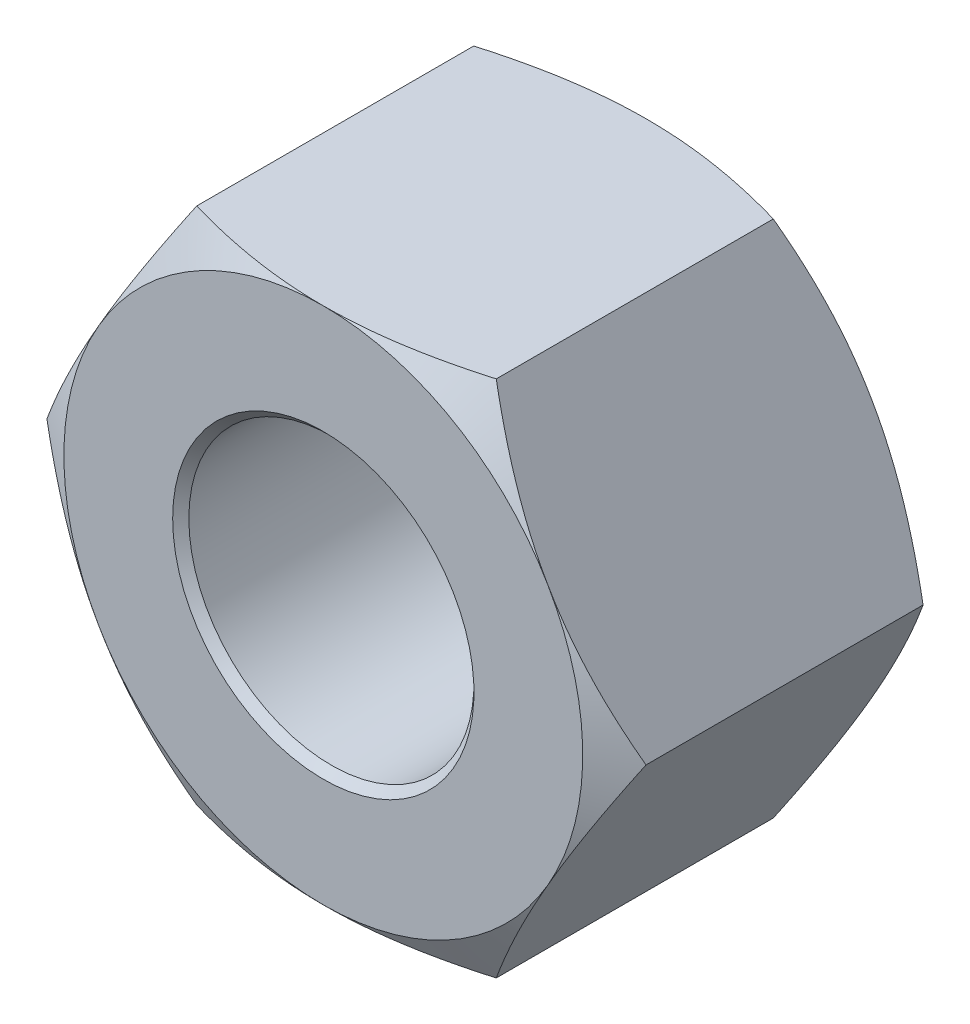
from build123d import *

# Parameters (mm, degrees)
SKETCH1_R          = 4.188125
BOSS_EXTRUDE_DEPTH = 9.5
SKETCH2_OUTSIDE_W  = 80.144
SKETCH2_OUTSIDE_H  = 77.786
SKETCH2_OUTSIDE_R  = 7.621023553
CUT_EXTRUDE1_DEPTH = 16.025644745
CUT_EXTRUDE1_DRAFT = -60
SKETCH3_OUTSIDE_W  = 80.144
SKETCH3_OUTSIDE_H  = 77.786
SKETCH3_OUTSIDE_R  = 7.621023553
CUT_EXTRUDE2_DEPTH = 16.025644745
CUT_EXTRUDE2_DRAFT = -60
CHAMFER1_SIZE      = 0.2375


with BuildPart() as part:
    # Sketch1 → Boss-Extrude (new body)
    with BuildSketch(Plane.XY):
        Polygon((4.4, 7.621023553), (-4.4, 7.621023553), (-8.8, 0), (-4.4, -7.621023553), (4.4, -7.621023553), (8.8, 0), align=None)
        Circle(SKETCH1_R, mode=Mode.SUBTRACT)
    extrude(amount=BOSS_EXTRUDE_DEPTH)


with BuildPart() as cut_extrude1_tool:
    # Sketch2 outside → Cut-Extrude1 (with draft: the straight prism first)
    with BuildSketch(Plane(origin=(0, 0, 0), x_dir=(-1, 0, 0), z_dir=(0, 0, -1))):
        Rectangle(SKETCH2_OUTSIDE_W, SKETCH2_OUTSIDE_H)
        Circle(SKETCH2_OUTSIDE_R, mode=Mode.SUBTRACT)
    extrude(amount=-CUT_EXTRUDE1_DEPTH)
    # Cut-Extrude1: the draft: its side faces are tilted about the plane it starts from
    cut_extrude1_sides = [cut_extrude1_tool.faces().sort_by_distance(p)[0] for p in [
        (0, -38.893, 8.012822372),
        (-40.072, 0, 8.012822372),
        (0, 38.893, 8.012822372),
        (40.072, 0, 8.012822372),
        (7.621023553, 0, 8.012822372),
    ]]
    draft(cut_extrude1_sides, Plane(origin=(0, 0, 0), x_dir=(-1, 0, 0), z_dir=(0, 0, -1)), CUT_EXTRUDE1_DRAFT)


with BuildPart() as part_1:
    add(part.part)

    # Cut-Extrude1: cut by cut_extrude1_tool
    add(cut_extrude1_tool.part, mode=Mode.SUBTRACT)


with BuildPart() as cut_extrude2_tool:
    # Sketch3 outside → Cut-Extrude2 (with draft: the straight prism first)
    with BuildSketch(Plane.XY.offset(9.5)):
        Rectangle(SKETCH3_OUTSIDE_W, SKETCH3_OUTSIDE_H)
        Circle(SKETCH3_OUTSIDE_R, mode=Mode.SUBTRACT)
    extrude(amount=-CUT_EXTRUDE2_DEPTH)
    # Cut-Extrude2: the draft: its side faces are tilted about the plane it starts from
    cut_extrude2_sides = [cut_extrude2_tool.faces().sort_by_distance(p)[0] for p in [
        (0, -38.893, 1.487177628),
        (40.072, 0, 1.487177628),
        (0, 38.893, 1.487177628),
        (-40.072, 0, 1.487177628),
        (-7.621023553, 0, 1.487177628),
    ]]
    draft(cut_extrude2_sides, Plane.XY.offset(9.5), CUT_EXTRUDE2_DRAFT)


with BuildPart() as part_2:
    add(part_1.part)

    # Cut-Extrude2: cut by cut_extrude2_tool
    add(cut_extrude2_tool.part, mode=Mode.SUBTRACT)

    # Chamfer1
    chamfer1_edges = [part_2.edges().sort_by_distance(p)[0] for p in [
        (-4.188125, 0, 0),
        (-4.188125, 0, 9.5),
    ]]
    chamfer(chamfer1_edges, length=CHAMFER1_SIZE)


solid = part_2.part
